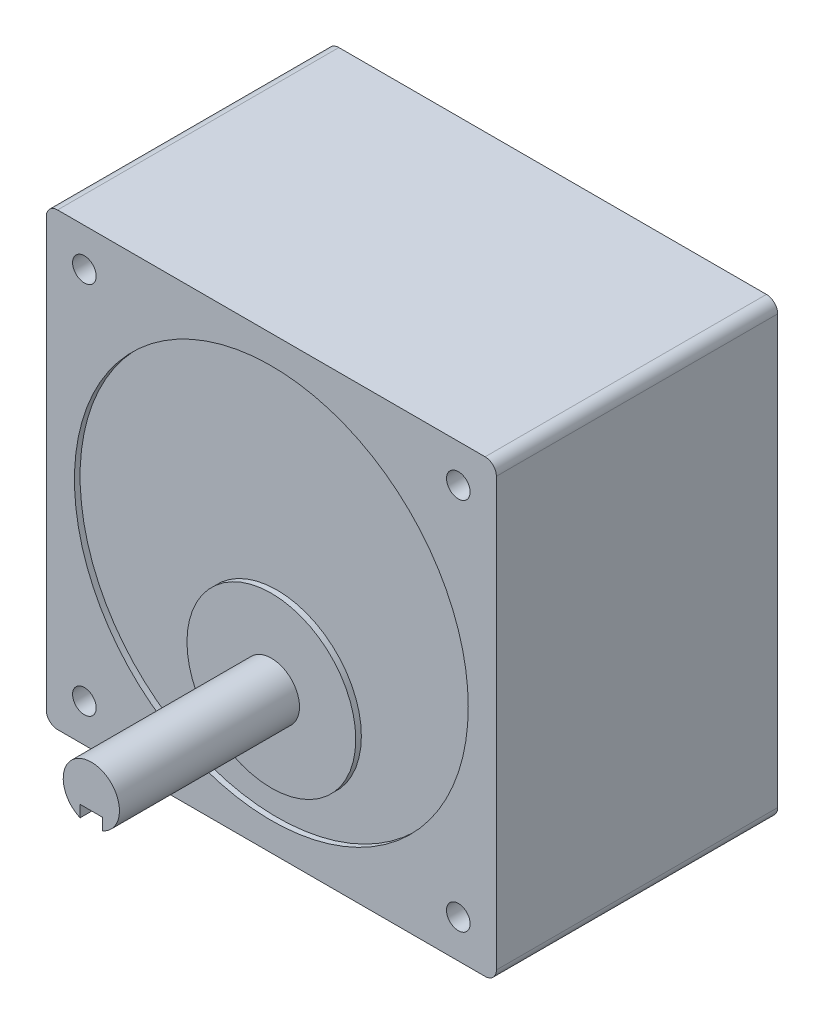
from build123d import *

# Parameters (mm, degrees)
SKETCH_1_W          = 80
SKETCH_1_H          = 80
EXTRUDE_1_DEPTH     = 50
SKETCH_2_R          = 35
CUT_EXTRUDE_1_DEPTH = 1
FILLET_1_R          = 2
HOLE_WIZARD_M5_1_D  = 4.2
SKETCH_10_R         = 5
CUT_EXTRUDE_2_DEPTH = 20
SKETCH_11_R         = 5
EXTRUDE_3_DEPTH     = 32
SKETCH_13_W         = 4
SKETCH_13_H         = 5
CUT_EXTRUDE_4_DEPTH = 25
SKETCH_14_R         = 15
EXTRUDE_4_DEPTH     = 1


with BuildPart() as part:
    # 草图1 → 凸台-拉伸1 (new body)
    with BuildSketch(Plane.XY):
        with Locations((40, 40)):
            Rectangle(SKETCH_1_W, SKETCH_1_H)
    extrude(amount=EXTRUDE_1_DEPTH)

    # 草图2 → 切除-拉伸1 (cut)
    with BuildSketch(Plane.XY.offset(50)):
        with Locations((40, 40)):
            Circle(SKETCH_2_R)
    extrude(amount=-CUT_EXTRUDE_1_DEPTH, mode=Mode.SUBTRACT)

    # 圆角1
    fillet_1_edges = [part.edges().sort_by_distance(p)[0] for p in [
        (0, 80, 25),
        (80, 80, 25),
        (80, 0, 25),
        (0, 0, 25),
    ]]
    fillet(fillet_1_edges, radius=FILLET_1_R)

    # M5 螺纹孔1 (through all)
    with Locations(Plane(origin=(73.234018716, 73.234018716, 0), x_dir=(-1, 0, 0), z_dir=(0, 0, -1))):
        with Locations((0, 0), (66.468037432, 0), (66.468037432, -66.468037432), (0, -66.468037432)):
            Hole(HOLE_WIZARD_M5_1_D / 2)

    # 草图10 → 切除-拉伸2 (cut)
    with BuildSketch(Plane(origin=(0, 0, 0), x_dir=(-1, 0, 0), z_dir=(0, 0, -1))):
        with Locations((-40, 40)):
            Circle(SKETCH_10_R)
    extrude(amount=-CUT_EXTRUDE_2_DEPTH, mode=Mode.SUBTRACT)



with BuildPart() as body_2:
    # 草图11 → 凸台-拉伸3 (new body)
    with BuildSketch(Plane.XY.offset(50)):
        with Locations((40, 25)):
            Circle(SKETCH_11_R)
    extrude(amount=EXTRUDE_3_DEPTH)

    # 草图13 → 切除-拉伸4 (cut)
    with BuildSketch(Plane.XY.offset(82)):
        with Locations((40, 20)):
            Rectangle(SKETCH_13_W, SKETCH_13_H)
    extrude(amount=-CUT_EXTRUDE_4_DEPTH, mode=Mode.SUBTRACT)


with BuildPart() as part_1:
    add(part.part)

    add(body_2.part)  # 凸台-拉伸4 merges body 2
    # 草图14 → 凸台-拉伸4 (add)
    with BuildSketch(Plane.XY.offset(49)):
        with Locations((40, 25)):
            Circle(SKETCH_14_R)
    extrude(amount=EXTRUDE_4_DEPTH)


solid = part_1.part
